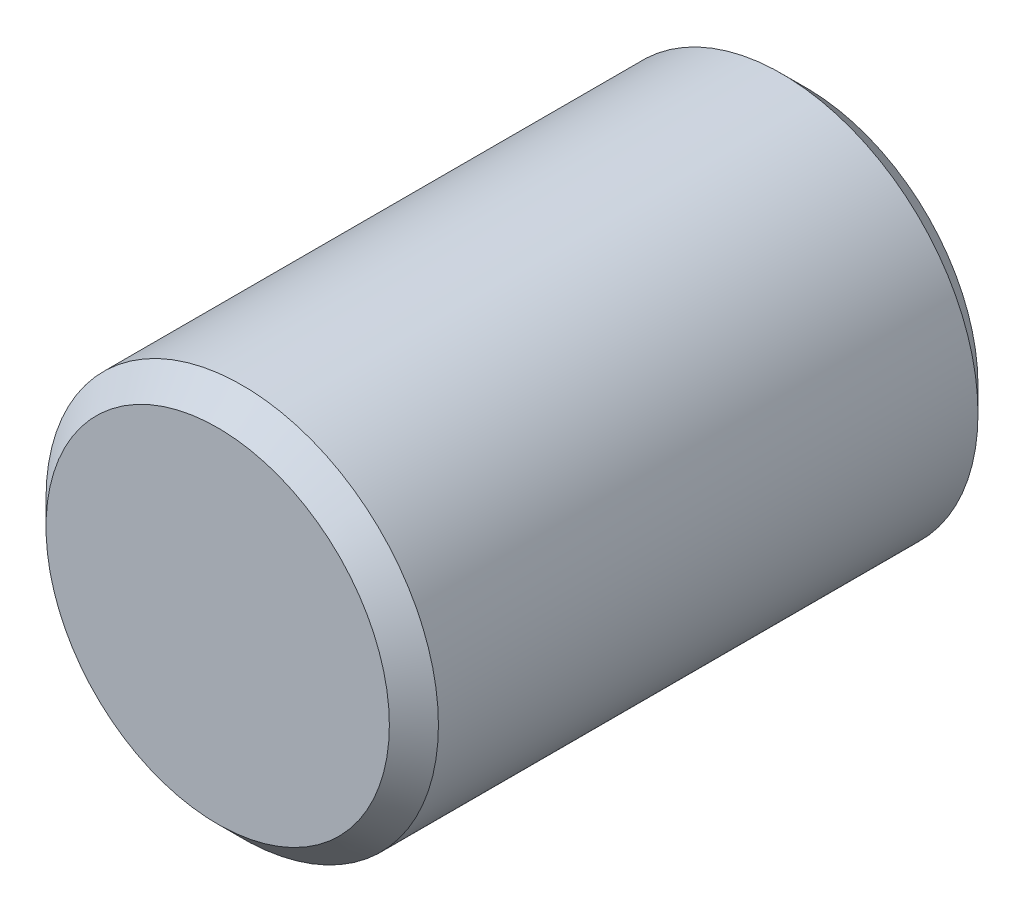
SolidWorks part; units mm, degrees
ref_plane "Front Plane" through (0, 0, 0) normal (0, 0, 1) x (1, 0, 0)
ref_plane "Top Plane" through (0, 0, 0) normal (0, 1, 0) x (1, 0, 0)
ref_plane "Right Plane" through (0, 0, 0) normal (1, 0, 0) x (0, 0, -1)
sketch "Sketch1" plane through (0, 0, 0) normal (0, 0, 1) x (1, 0, 0)
  circle A0 centre (0, 0) radius 4
  dimension "D1" = 8
extrude "Boss-Extrude1" add sketch "Sketch1" along normal blind 12
chamfer "Chamfer1" distance 0.5 angle 45 2 edges at (4, 0, 0) (4, 0, 12)
